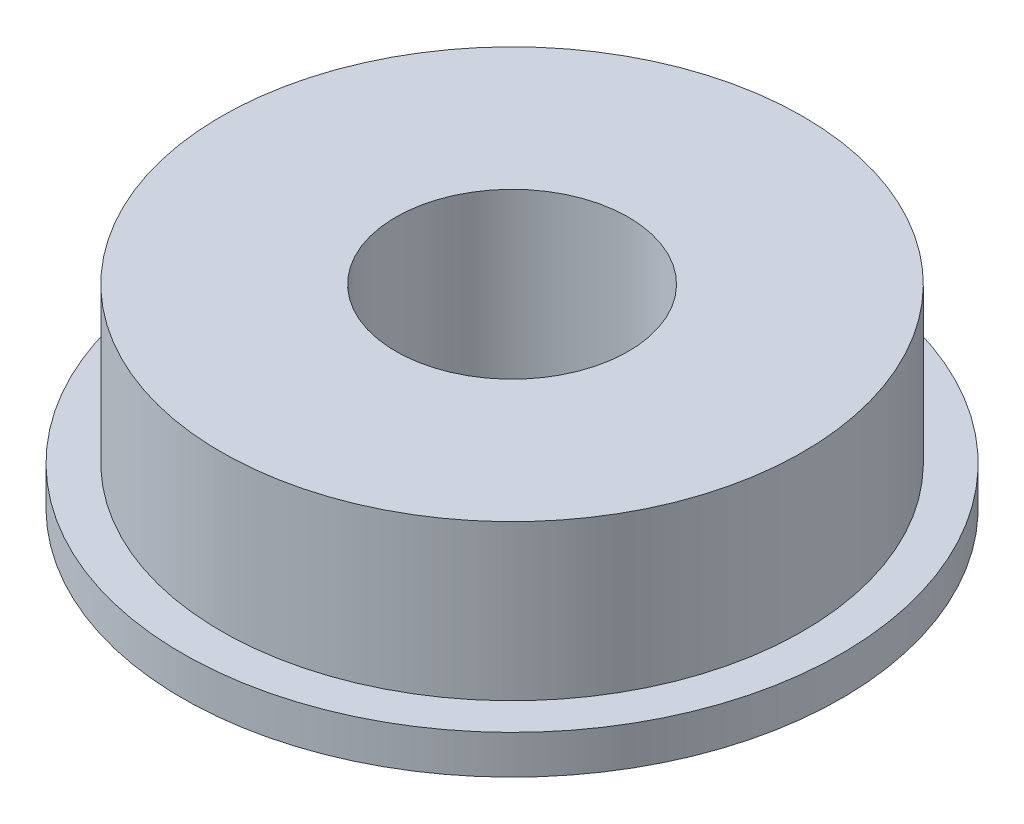
SolidWorks part; units mm, degrees
ref_plane "前视基准面" through (0, 0, 0) normal (0, 0, 1) x (1, 0, 0)
ref_plane "上视基准面" through (0, 0, 0) normal (0, 1, 0) x (1, 0, 0)
ref_plane "右视基准面" through (0, 0, 0) normal (1, 0, 0) x (0, 0, -1)
sketch "草图1" plane through (0, 0, 0) normal (0, 0, 1) x (1, 0, 0)
  line L0 (0, 0) -> (0, 5146.76) construction
  line L1 (3, 2.3174) -> (7.5, 2.3174)
  line L2 (7.5, 2.3174) -> (7.5, -1.6826)
  line L3 (7.5, -1.6826) -> (8.5, -1.6826)
  line L4 (8.5, -1.6826) -> (8.5, -2.6826)
  line L5 (8.5, -2.6826) -> (3, -2.6826)
  line L6 (3, -2.6826) -> (3, 2.3174)
  dimension "D1" = 3
  dimension "D2" = 5
  dimension "D3" = 5.5
  dimension "D4" = 4.5
  dimension "D5" = 1
revolve "旋转1" add sketch "草图1" angle 360 about L0
